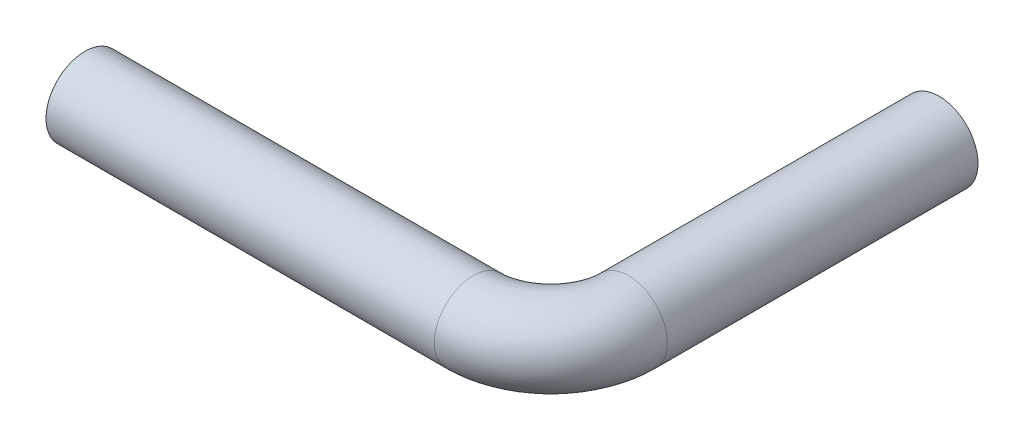
from build123d import *

# Parameters (mm, degrees)
SKETCH1_R   = 2.5
SKETCH1_R_2 = 2


with BuildPart() as part:
    # Sweep1: sweep along a path in Sketch2
    with BuildLine(Plane(origin=(0, 0, 0), x_dir=(1, 0, 0), z_dir=(0, 1, 0))) as sweep1_path:
        Line((0, 0), (0, -20))
        ThreePointArc((0, -20), (-1.464466094, -23.535533906), (-5, -25))
        Line((-5, -25), (-30, -25))
    # Sketch1 → Sweep1 (sweep)
    with BuildSketch(Plane.XY):
        Circle(SKETCH1_R)
        Circle(SKETCH1_R_2, mode=Mode.SUBTRACT)
    sweep(path=sweep1_path.line)


solid = part.part
